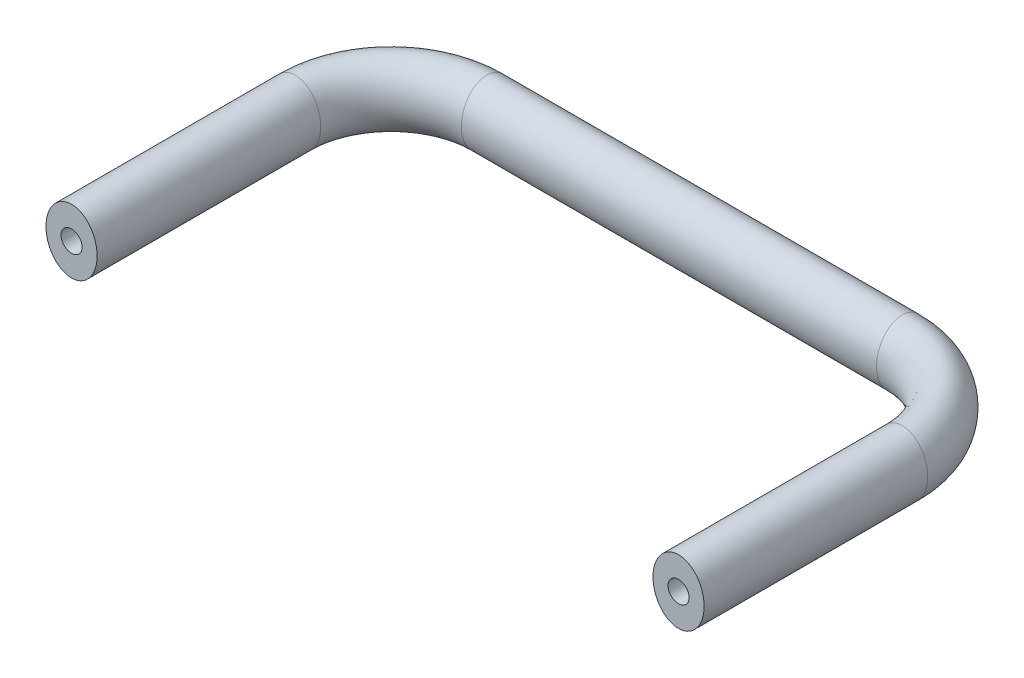
from build123d import *

# Parameters (mm, degrees)
SKETCH_1_RX            = 5
SKETCH_1_RY            = 4
HOLE_WIZARD_M4_1_D     = 3.3
HOLE_WIZARD_M4_1_DEPTH = 11.5
HOLE_WIZARD_M4_1_TIP   = 0.991420021


with BuildPart() as part:
    # 扫描1: sweep along a path in 草图2
    with BuildLine(Plane(origin=(0, 0, 0), x_dir=(1, 0, 0), z_dir=(0, 1, 0))) as sweep_1_path:
        Line((0, 0), (0, 35))
        ThreePointArc((0, 35), (4.393398282, 45.606601718), (15, 50))
        Line((15, 50), (80, 50))
        ThreePointArc((80, 50), (90.606601718, 45.606601718), (95, 35))
        Line((95, 35), (95, 0))
    # 草图1 → 扫描1 (sweep)
    with BuildSketch(Plane.XY):
        with Locations(Location((0, 0), (0, 0, 90))):
            Ellipse(SKETCH_1_RX, SKETCH_1_RY)
    sweep(path=sweep_1_path.line)

    # M4 螺纹孔1
    with Locations(Plane.XY):
        with Locations((0, 0), (95, 0)):
            Hole(HOLE_WIZARD_M4_1_D / 2, depth=HOLE_WIZARD_M4_1_DEPTH)
            with Locations((0, 0, -(HOLE_WIZARD_M4_1_DEPTH + HOLE_WIZARD_M4_1_TIP / 2))):  # 118° drill point
                Cone(0, HOLE_WIZARD_M4_1_D / 2, HOLE_WIZARD_M4_1_TIP, mode=Mode.SUBTRACT)


solid = part.part
